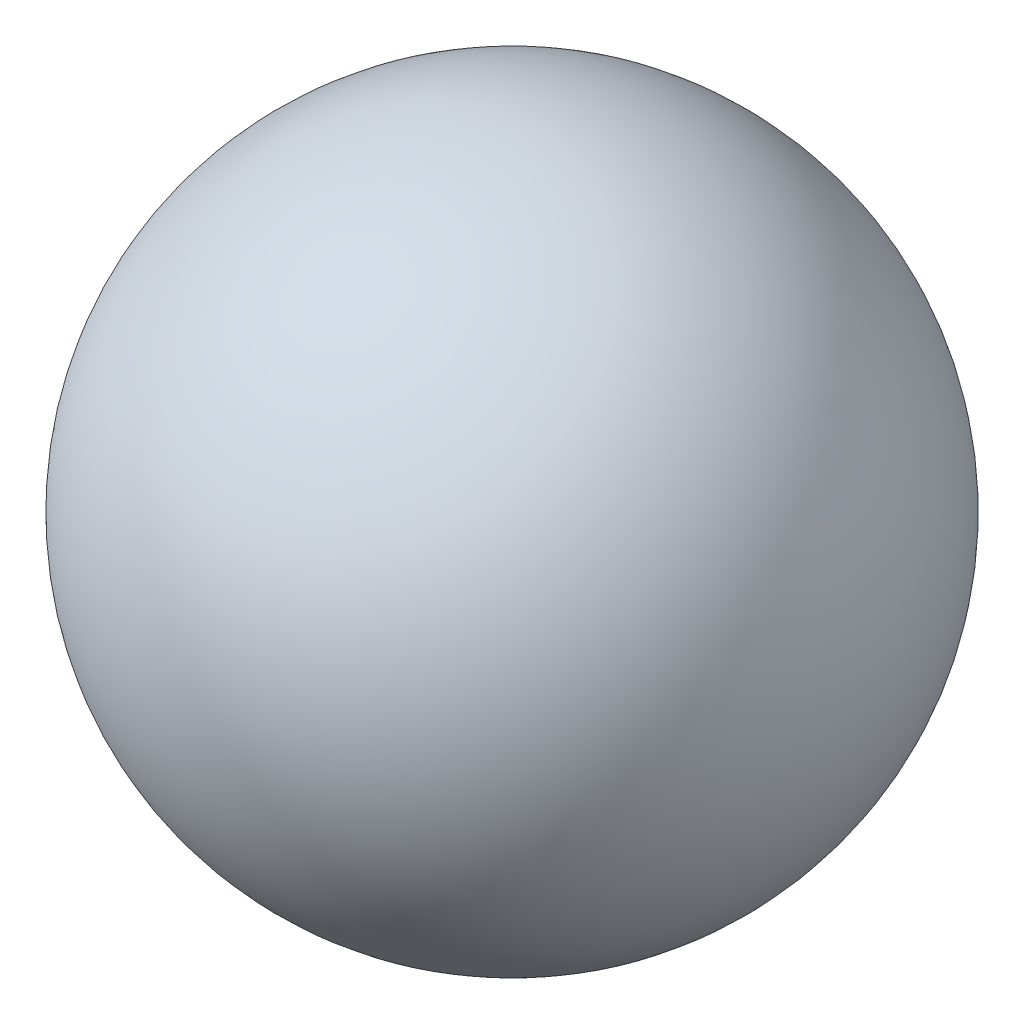
from build123d import *


with BuildPart() as part:
    # 草图1 → 旋转1 (revolve)
    with BuildSketch(Plane.XY):
        with BuildLine():
            Line((0, 25), (0, -25))
            ThreePointArc((0, -25), (25, 0), (0, 25))
        make_face()
    revolve(axis=Axis((0, 25, 0), (0, -1, 0)))


solid = part.part
